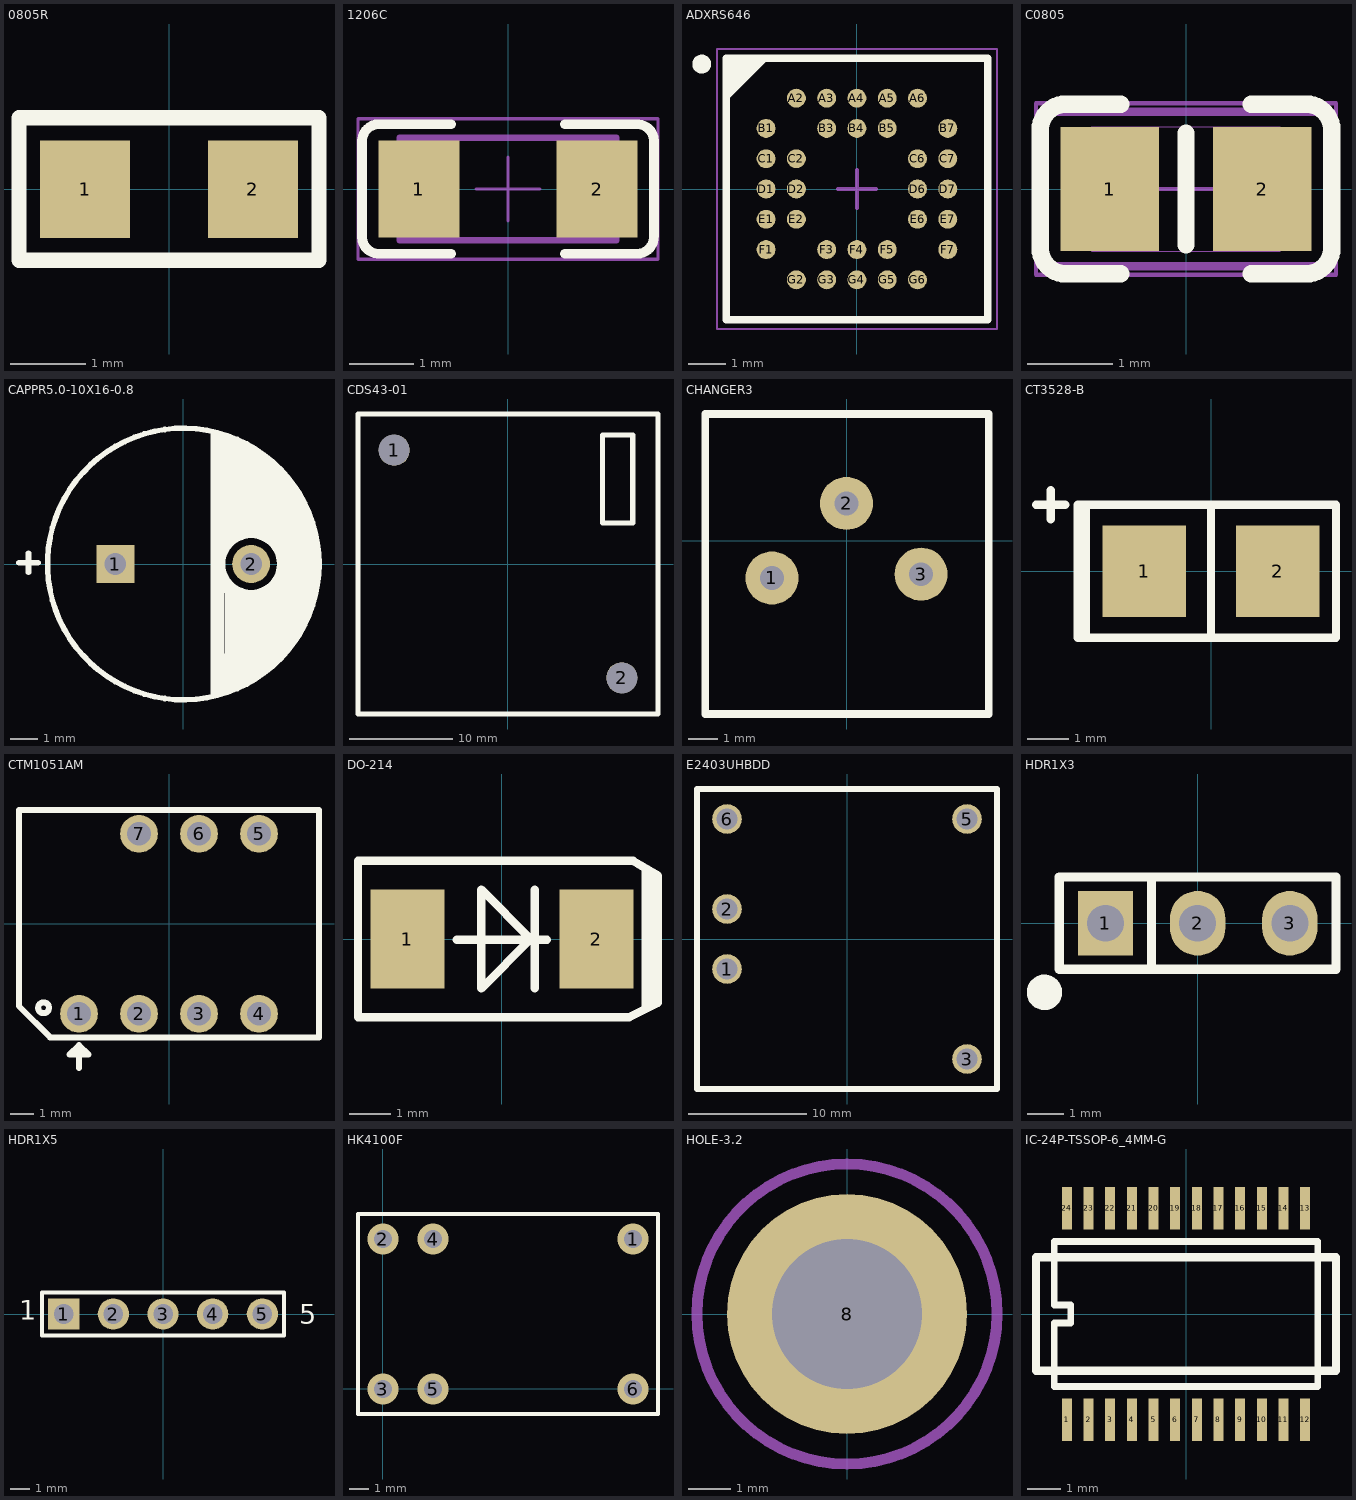
[diagram p0: the footprints below, top view; thin cyan lines are the x and y axes]
# Altium footprint library MISC82155.PcbLib: 38 footprints (part 1 of 3)
Each footprint in its own frame and in the unit in brackets; x right, y up, seen from the top. Pads: shape width x height; smd on the part's side, far side on the other; paste and mask are expansions set on the pad; w line width, h text height; cw(c..) or ccw(c..) is an arc to the next point about the centre after c.

## 0805R [mm]
height 1.2
pads (2):
  rect 1.2x1.3 smd: 1(-1.118,0) 2(1.118,0)
Top Overlay:
  lines w0.203: -2,-0.95 2,-0.95 2,0.95 -2,0.95 -2,-0.95

## 1206C [mil]
height 40
pads (2):
  rect 50x60 smd: 1(-55,0) 2(55,0)
Top Overlay:
  lines w6: -90,29 cw(c-79.5,29.5) -80,40 -35,40 ; -90,30 -90,-30 ccw(c-79.5,-29.5) -79,-40 ; -80,-40 -35,-40 ; 35,-40 79,-40 ; 35,40 80,40 ; 79,40 cw(c79.5,29.5) 90,30 90,-29 cw(c79.5,-29.5) 80,-40
Mechanical 15:
  lines w3.94: -66.93,-31.5 -66.93,31.5 66.93,31.5 66.93,-31.5 -66.93,-31.5
  text "1" at -6.47,-17.71 h40
Mechanical 16:
  lines w0.04: -66.93,-31.5 -66.93,31.5 66.93,31.5 66.93,-31.5 -66.93,-31.5
  lines w1.97: -19.68,0 19.68,0 ; 0,-19.68 0,19.68 ; -92.52,-43.31 -92.52,43.31 92.52,43.31 92.52,-43.31 -92.52,-43.31
3D body: height 39.37, standoff 0, extent -62,-32 63.98,30.99

## ADXRS646 [mm] "BGA, 32-Leads, Body 6.88x6.88mmx3.80mm, Pitch 0.80mm"
height 3.8
pads (32):
  round 0.5 smd: A2(-1.6,2.4) A3(-0.8,2.4) A4(0,2.4) A5(0.8,2.4) A6(1.6,2.4) B1(-2.4,1.6) B3(-0.8,1.6) B4(0,1.6) B5(0.8,1.6) B7(2.4,1.6) C1(-2.4,0.8) C2(-1.6,0.8) C6(1.6,0.8) C7(2.4,0.8) D1(-2.4,0) D2(-1.6,0) D6(1.6,0) D7(2.4,0) E1(-2.4,-0.8) E2(-1.6,-0.8) E6(1.6,-0.8) E7(2.4,-0.8) F1(-2.4,-1.6) F3(-0.8,-1.6) F4(0,-1.6) F5(0.8,-1.6) F7(2.4,-1.6) G2(-1.6,-2.4) G3(-0.8,-2.4) G4(0,-2.4) G5(0.8,-2.4) G6(1.6,-2.4)
Top Overlay:
  circle w0.25: c-4.1,3.3 r0.125
  region: -2.45,3.45 -3.45,2.45 -3.45,3.45
  lines w0.2: -3.45,2.45 -2.45,3.45 ; -3.45,-3.45 -3.45,3.45 3.45,3.45 3.45,-3.45 -3.45,-3.45
Mechanical 13:
  lines w0.1: -3.44,-3.44 -3.44,3.44 3.44,3.44 3.44,-3.44 -3.44,-3.44
Mechanical 15:
  lines w0.05: -3.7,-3.7 -3.7,3.7 3.7,3.7 3.7,-3.7 -3.7,-3.7
  lines w0.1: -0.5,0 0.5,0 ; 0,-0.5 0,0.5
3D body: height 3.8, standoff 0.5, extent -3.44,-3.44 3.44,3.44

## C0805 [mm] "Chip Capacitor, Body 2.0x1.3mm, IPC High Density"
height 1.4
pads (2):
  rect 1.15x1.45 smd: 1(-0.889,0) 2(0.889,0)
Top Overlay:
  lines w0.2: 0,-0.65 0,0.65
  lines w0.203: -0.762,-0.991 -1.397,-0.991 cw(c-1.397,-0.686) -1.702,-0.686 -1.702,0.686 cw(c-1.397,0.686) -1.397,0.991 -0.762,0.991 ; 0.762,-0.991 1.397,-0.991 ccw(c1.397,-0.686) 1.702,-0.686 1.702,0.686 ccw(c1.397,0.686) 1.397,0.991 0.762,0.991
Mechanical 15:
  lines w0.1: -1.65,-0.9 1.65,-0.9 1.65,0.9 -1.65,0.9 -1.65,-0.9
  text "1" at -0.164,-0.45 h1.27
Mechanical 16:
  lines w0.001: -1.1,-0.725 1.1,-0.725 1.1,0.725 -1.1,0.725 -1.1,-0.725
  lines w0.05: -0.5,0 0.5,0 ; 0,-0.5 0,0.5 ; -1.75,-1 1.75,-1 1.75,1 -1.75,1 -1.75,-1
3D body: height 0.78, standoff 0, extent -1,-0.625 1,0.625

## CAPPR5.0-10X16-0.8 [mm]
pads (2):
  rect 1.4x1.4 hole 0.8: 1(-2.5,0)
  round 1.4 hole 0.8: 2(2.5,0)
Top Overlay:
  circle w0.5: c2.5,0 r1.2
  circle w0.203: c0,0 r5
  rectangle: 1,-4.8 1.4,4.8
  rectangle: 1.3,-4.71 1.5,4.79
  rectangle: 1.45,1.01 2.8,4.21
  rectangle: 2.7,1 3.5,3.6
  rectangle: 3.49,-3.2 3.79,3.3
  rectangle: 1.51,-3.5 3.51,-1
  rectangle: 1.5,-4.2 2.8,-3.3
  rectangle: 3.7,-2.61 4.2,2.79
  rectangle: 4.1,-1.8 4.6,2.2
  rectangle: 4.5,-1.1 4.9,1.4
  lines w0.203: -6.05,0.05 -5.7,0.05 ; -5.7,-0.3 -5.7,0.05 ; -5.7,0.4 -5.7,0.05 ; -5.35,0.05 -5.7,0.05
  lines w1: 1.514,-4.238 ccw(c0,0) 1.569,4.217
3D body: height 15.68, standoff -2.45, extent -5.1,-5.1 4.9,4.9

## CDS43-01 [mm]
height 9.5
pads (2):
  round 3 hole 3: 1(-11,11) 2(11,-11)
Top Overlay:
  lines w0.5: -14.5,-14.5 -14.5,14.5 14.5,14.5 14.5,-14.5 -14.5,-14.5 ; 9.129,3.962 9.129,12.467 12.053,12.467 12.053,3.962 9.129,3.962

## CHANGER3 [mm]
height 9.5
pads (3):
  round 1.778 hole 0.8: 1(-2.5,-1.25) 2(0,1.25) 3(2.5,-1.123)
Top Overlay:
  lines w0.254: -4.734,-5.811 -4.734,4.25 4.766,4.25 4.766,-5.811 -4.734,-5.811

## CT3528-B [mm]
height 3.98
pads (2):
  rect 2x2.2 smd: 1(-1.6,0) 2(1.6,0)
Top Overlay:
  rectangle: -3.2,-1.5 -2.9,1.5
  lines w0.203: -4.2,1.6 -3.85,1.6 ; -3.85,1.25 -3.85,1.6 ; -3.85,1.95 -3.85,1.6 ; -3.5,1.6 -3.85,1.6 ; 0,-1.6 0,1.5 ; -3.2,-1.6 -3.2,1.6 3,1.6 3,-1.6 -3.2,-1.6
3D body: height 1.9, standoff 0, extent -1.75,-1.4 1.75,1.4

## CTM1051AM [mm]
pads (7):
  round 1.6 hole 1: 1(-3.81,-3.81) 2(-1.27,-3.81) 3(1.27,-3.81) 4(3.81,-3.81) 5(3.81,3.81) 6(1.27,3.81) 7(-1.27,3.81)
Top Overlay:
  circle w0.254: c-5.31,-3.556 r0.23
  lines w0.254: -3.81,-6.096 -3.81,-5.131 ; -3.81,-5.131 -4.216,-5.537 -3.404,-5.537 -3.81,-5.131 ; -6.35,-3.489 -5.029,-4.81 6.35,-4.81 6.35,4.81 -6.35,4.81 -6.35,-3.489

## DO-214 [mm]
height 9.5
pads (2):
  rect 1.8x2.4 smd: 1(-2.3,0) 2(2.3,0)
Top Overlay:
  lines w0.203: -1.1,-0.02 1.1,-0.02 ; 0.8,-1.2 0.8,1.2 ; 3.5,-1.7 3.5,1.7 ; 3.7,-1.5 3.7,1.6 ; -3.5,-1.9 3.1,-1.9 3.8,-1.55 3.8,1.54 3.2,1.9 -3.5,1.9 -3.5,-1.9 ; -0.5,-1.2 0.7,0 -0.5,1.2 -0.5,-1.2

## E2403UHBDD [mm]
height 9.5
pads (5):
  round 2.5 hole 1.8: 1(-10.16,-2.54) 2(-10.16,2.54) 3(10.16,-10.16) 5(10.16,10.16) 6(-10.16,10.16)
Top Overlay:
  lines w0.5: -12.7,-12.7 12.7,-12.7 12.7,12.7 -12.7,12.7 -12.7,-12.7

## HDR1X3 [mil]
height 374.02
pads (3):
  rect 60x70 hole 40: 1(-100,0)
  oval 60x70 hole 40: 2(0,0) 3(100,0)
Top Overlay:
  circle w20: c-166.11,-75 r9.22
  lines w10: -50,-50 -50,50 ; -150,-50 150,-50 150,50 -150,50 -150,-50
3D body: height 298.43, standoff -115.75, extent 50,-50 150,50
3D body: height 298.43, standoff -115.75, extent -150,-50 -50,50
3D body: height 298.43, standoff -115.75, extent -50,-50 50,50

## HDR1X5 [mm]
height 9.5
pads (5):
  rect 1.6x1.6 hole 1: 1(-5.08,0)
  round 1.6 hole 1: 2(-2.54,0) 3(0,0) 4(2.54,0) 5(5.08,0)
Top Overlay:
  lines w0.203: -6.18,-1.1 6.18,-1.1 6.18,1.1 -6.18,1.1 -6.18,-1.1
  text "1" at -7.366,-0.305 h1.02
  text "5" at 6.96,-0.508 h1.02

## HK4100F [mm]
height 9.5
pads (6):
  round 1.6 hole 0.9: 1(12.7,7.62) 2(0,7.62) 3(0,0) 4(2.54,7.62) 5(2.54,0) 6(12.7,0)
Top Overlay:
  lines w0.2: -1.27,-1.27 13.97,-1.27 13.97,8.89 -1.27,8.89 -1.27,-1.27

## HOLE-3.2 [mm]
height 9.5
pads (1):
  round 5.6 hole 3.5: 8(0,0)
Mechanical 15:
  circle w0.254: c0,0 r3.5

## IC-24P-TSSOP-6_4MM-G [mm]
pads (24):
  rect 0.305x1.27 smd: 1(-3.575,-3.175) 2(-2.925,-3.175) 3(-2.275,-3.175) 4(-1.625,-3.175) 5(-0.975,-3.175) 6(-0.325,-3.175) 7(0.325,-3.175) 8(0.975,-3.175) 9(1.625,-3.175) 10(2.275,-3.175) 11(2.925,-3.175) 12(3.575,-3.175) 13(3.575,3.175) 14(2.925,3.175) 15(2.275,3.175) 16(1.625,3.175) 17(0.975,3.175) 18(0.325,3.175) 19(-0.325,3.175) 20(-0.975,3.175) 21(-1.625,3.175) 22(-2.275,3.175) 23(-2.925,3.175) 24(-3.575,3.175)
Top Overlay:
  lines w0.203: -3.95,-2.175 -3.95,-0.272 -3.456,-0.272 -3.456,0.272 -3.95,0.272 -3.95,2.175 3.95,2.175 3.95,-2.175 -3.95,-2.175
  lines w0.254: -4.5,-1.7 4.5,-1.7 4.5,1.7 -4.5,1.7 -4.5,-1.7